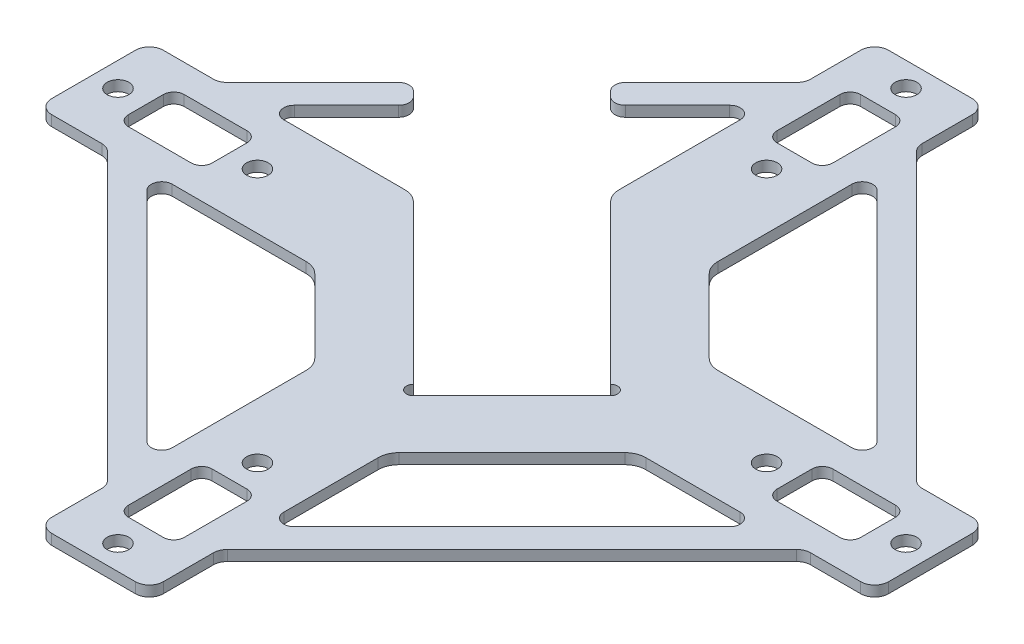
SolidWorks part; units mm, degrees
material "Thornel Mat VMA"
ref_plane "前视基准面" through (0, 0, 0) normal (0, 0, 1) x (1, 0, 0)
ref_plane "上视基准面" through (0, 0, 0) normal (0, 1, 0) x (1, 0, 0)
ref_plane "右视基准面" through (0, 0, 0) normal (1, 0, 0) x (0, 0, -1)
other "Configuration Table"
sketch "草图1" plane through (0, 0, 0) normal (0, 1, 0) x (1, 0, 0)
  line L0 (0, 0) -> (48.5733, 0) construction
  line L1 (0, 0) -> (0, 54.2635) construction
  line L2 (-8, 60) -> (8, 60)
  line L3 (60, 8) -> (60, -8)
  line L4 (8, -60) -> (-8, -60)
  line L5 (-60, -8) -> (-60, 8)
  line L6 (8, 60) -> (8, 14.6274)
  line L7 (0, 0) -> (59.1939, 59.1939) construction
  line L8 (8, 14.6274) -> (11.3137, 11.3137)
  line L9 (60, 8) -> (14.6274, 8)
  line L10 (14.6274, 8) -> (11.3137, 11.3137)
  line L11 (4, 52.5) -> (4, 40.5)
  line L12 (-52.5, 4) -> (-40.5, 4)
  line L13 (60, -8) -> (14.6274, -8)
  line L14 (8, -60) -> (8, -14.6274)
  line L15 (8, -14.6274) -> (14.6274, -8)
  line L16 (-8, -60) -> (-8, -14.6274)
  line L17 (-8, -14.6274) -> (-14.6274, -8)
  line L18 (-60, -8) -> (-14.6274, -8)
  line L19 (-60, 8) -> (-60, -8)
  line L20 (-60, 8) -> (-14.6274, 8)
  line L21 (-8, 14.6274) -> (-11.3137, 11.3137)
  line L22 (-14.6274, 8) -> (-11.3137, 11.3137)
  line L23 (-8, 60) -> (-8, 14.6274)
  line L24 (8, 44.3431) -> (44.3431, 8)
  line L25 (8, 50) -> (50, 8)
  line L26 (-8, 44.3431) -> (-44.3431, 8)
  line L27 (-8, 50) -> (-50, 8)
  line L28 (8, -50) -> (50, -8)
  line L29 (8, -44.3431) -> (44.3431, -8)
  line L30 (-8, -44.3431) -> (-44.3431, -8)
  line L31 (-8, -50) -> (-50, -8)
  line L32 (-52.5, 4) -> (-52.5, -4)
  line L33 (-52.5, -4) -> (-40.5, -4)
  line L34 (-40.5, 4) -> (-40.5, -4)
  line L35 (-52.5, 4) -> (-40.5, -4) construction
  line L36 (-52.5, -4) -> (-40.5, 4) construction
  line L37 (4, 52.5) -> (-4, 52.5)
  line L38 (-4, 52.5) -> (-4, 40.5)
  line L39 (4, 40.5) -> (-4, 40.5)
  line L40 (4, 52.5) -> (-4, 40.5) construction
  line L41 (-4, 52.5) -> (4, 40.5) construction
  line L42 (52.5, -4) -> (40.5, -4)
  line L43 (52.5, -4) -> (52.5, 4)
  line L44 (52.5, 4) -> (40.5, 4)
  line L45 (40.5, -4) -> (40.5, 4)
  line L46 (52.5, -4) -> (40.5, 4) construction
  line L47 (52.5, 4) -> (40.5, -4) construction
  line L48 (-4, -52.5) -> (-4, -40.5)
  line L49 (-4, -52.5) -> (4, -52.5)
  line L50 (4, -52.5) -> (4, -40.5)
  line L51 (-4, -40.5) -> (4, -40.5)
  line L52 (-4, -52.5) -> (4, -40.5) construction
  line L53 (4, -52.5) -> (-4, -40.5) construction
  line L54 (-20.2843, -8) -> (-8, -20.2843)
  line L55 (8, 20.2843) -> (20.2843, 8)
  line L67 (-36.0711, 21.9289) -> (-33.2426, 19.1005)
  line L68 (0, 0) -> (-29, 29) construction
  line L69 (-21.9289, 36.0711) -> (-19.1005, 33.2426)
  line L70 (-33.2426, 19.1005) -> (2.8284, -16.9706)
  line L71 (-19.1005, 33.2426) -> (16.9706, -2.8284)
  line L72 (2.8284, -16.9706) -> (16.9706, -2.8284)
  line L73 (8, -25.9411) -> (25.9411, -8)
  circle A0 centre (0, 0) radius 7.5
  circle A1 centre (0, 56.5) radius 1.55
  circle A2 centre (56.5, 0) radius 1.55
  circle A3 centre (0, -56.5) radius 1.55
  circle A4 centre (-56.5, 0) radius 1.55
  circle A7 centre (0, 36.5) radius 1.55
  circle A8 centre (36.5, 0) radius 1.55
  circle A9 centre (0, -36.5) radius 1.55
  circle A10 centre (-36.5, 0) radius 1.55
  circle A11 centre (16.2635, -2.1213) radius 1
  circle A13 centre (2.1213, -16.2635) radius 1
  point P4 (-46.5, 0)
  point P24 (0, 0)
  point P53 (0, 0)
  point P69 (0, 46.5)
  point P74 (46.5, 0)
  point P79 (0, -46.5)
  point P84 (0, 0)
  point P163 (0, 0)
  dimension "D1" = 15
  dimension "D3" = 3.1
  dimension "D4" = 3.5
  dimension "D8" = 16
  dimension "D12" = 4
  dimension "D13" = 20
  dimension "D18" = 2
  dimension "D11" = 10
  dimension "D17" = 10
  dimension "D2" = 16
  dimension "D5" = 60
  dimension "D7" = 45
  dimension "D9" = 8
  dimension "D10" = 12
  dimension "D15" = 4
  dimension "D16" = 10
  dimension "D19" = 10
  dimension "D34" = 20
  dimension "D35" = 14
  dimension "D36" = 10
  dimension "D6" = 4
  dimension "D14" = 4
extrude "凸台-拉伸1" add sketch "草图1" along normal blind 1.5
sketch "草图2" plane through (0, 1.5, 0) normal (0, 1, 0) x (1, 0, 0)
  line L0 (-19.3137, 5.1716) -> (-16.4853, 2.3431)
  line L1 (-19.3137, 5.1716) -> (-5.1716, 19.3137)
  line L2 (-16.4853, 2.3431) -> (-2.3431, 16.4853)
  line L3 (-5.1716, 19.3137) -> (-2.3431, 16.4853)
  line L4 (-22.1421, 8) -> (1.4142, -15.5563) construction
  line L5 (-8, 22.1421) -> (15.5563, -1.4142) construction
  dimension "D1" = 4
  dimension "D2" = 4
extrude "凸台-拉伸2" [suppressed] add sketch "草图2" against normal up to surface (1.5 mm away)
fillet "2mm" radius 2 16 edges at (-50, 0.75, -8) (-60, 0.75, -8) (-60, 0.75, 8) (-50, 0.75, 8) (-8, 0.75, 50) (-8, 0.75, 60) (8, 0.75, 60) (8, 0.75, 50) (50, 0.75, 8) (60, 0.75, 8) (60, 0.75, -8) (50, 0.75, -8) (8, 0.75, -50) (8, 0.75, -60) (-8, 0.75, -50) (-8, 0.75, -60)
fillet "1.5mm" radius 1.5 28 edges at (-21.9289, 0.75, -36.0711) (-19.1005, 0.75, -33.2426) (-36.0711, 0.75, -21.9289) (-33.2426, 0.75, -19.1005) (-44.3431, 0.75, -8) (-8, 0.75, -44.3431) (-52.5, 0.75, -4) (-52.5, 0.75, 4) (-40.5, 0.75, -4) (-40.5, 0.75, 4) (-44.3431, 0.75, 8) (-8, 0.75, 44.3431) (-4, 0.75, 52.5) (4, 0.75, 40.5) (-4, 0.75, 40.5) (4, 0.75, 52.5) (8, 0.75, 44.3431) (44.3431, 0.75, 8) (8, 0.75, -44.3431) (44.3431, 0.75, -8) (4, 0.75, -52.5) (-4, 0.75, -52.5) (-4, 0.75, -40.5) (4, 0.75, -40.5) (52.5, 0.75, 4) (52.5, 0.75, -4) (40.5, 0.75, 4) (40.5, 0.75, -4)
fillet "3mm" radius 3 8 edges at (-22.1421, 0.75, -8) (-8, 0.75, -22.1421) (25.9411, 0.75, 8) (8, 0.75, 25.9411) (20.2843, 0.75, -8) (8, 0.75, -20.2843) (-8, 0.75, 20.2843) (-20.2843, 0.75, 8)
